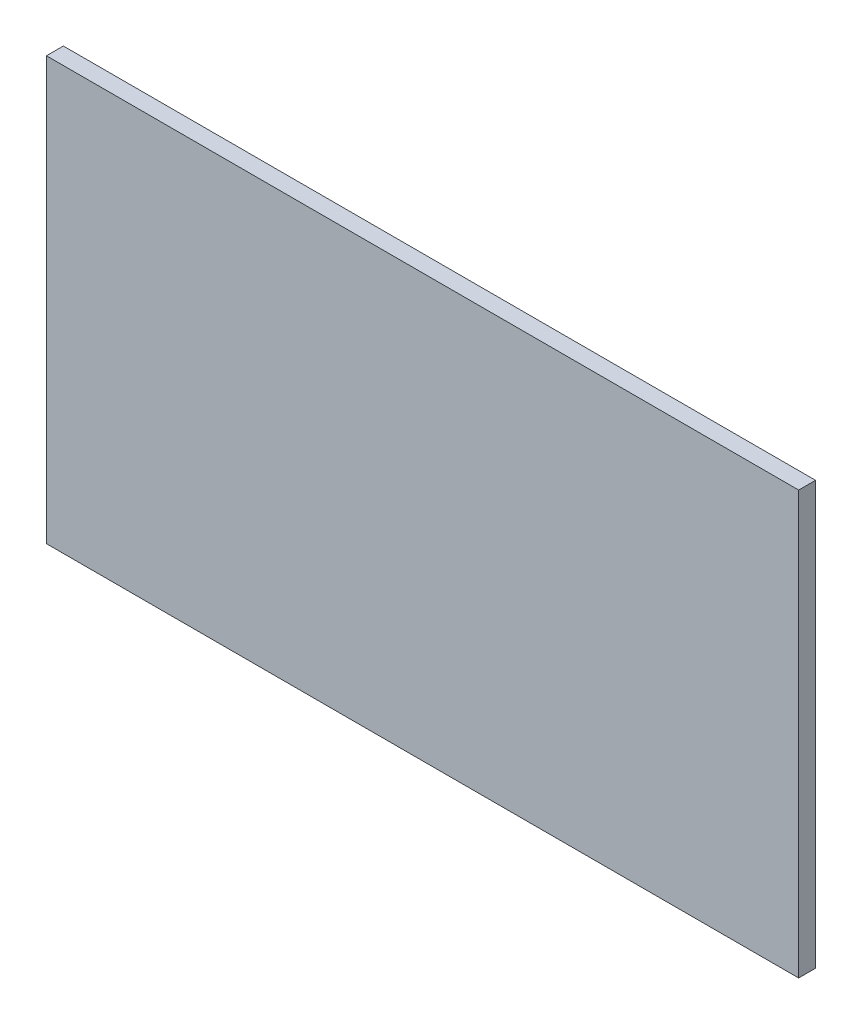
from build123d import *

# Parameters (mm, degrees)
BOSS_EXTRUDE1_DEPTH = 40


with BuildPart() as part:
    # Sketch1 → Boss-Extrude1 (new body)
    with BuildSketch(Plane.XY):
        Polygon((0, 0), (0, 1000), (1780, 1000), (1780, 500), (1780, 0), align=None)
    extrude(amount=BOSS_EXTRUDE1_DEPTH)


solid = part.part
